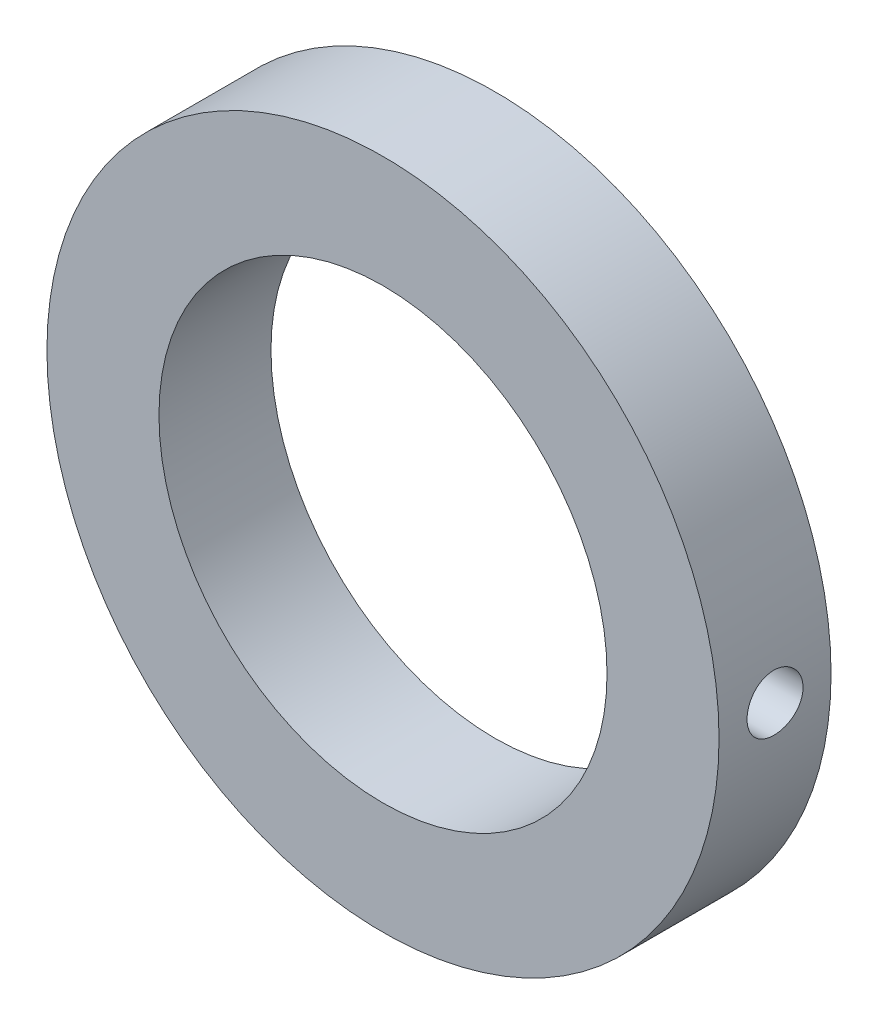
SolidWorks part; units mm, degrees
ref_plane "前视基准面" through (0, 0, 0) normal (0, 0, 1) x (1, 0, 0)
ref_plane "上视基准面" through (0, 0, 0) normal (0, 1, 0) x (1, 0, 0)
ref_plane "右视基准面" through (0, 0, 0) normal (1, 0, 0) x (0, 0, -1)
sketch "草图1" plane through (0, 0, 0) normal (0, 0, 1) x (1, 0, 0)
  circle A0 centre (0, 0) radius 10
  circle A1 centre (0, 0) radius 15
  dimension "D1" = 20
  dimension "D2" = 30
extrude "凸台-拉伸1" add sketch "草图1" along normal blind 5
hole_wizard "M3 螺纹孔2" positions "3D草图2" profile "草图3" tap size "M3" standard "Iso"
sketch3d "3D草图2"
  point P0 (14.9997, 0.1016, 2.5)
sketch "草图3" plane through (14.9997, 0.1016, 2.5) normal (0, 0, 1) x (-0.0068, 1, 0)
  line L0 (0, 0) -> (0, 8.2511)
  line L1 (0, 8.2511) -> (1.25, 7.5)
  line L2 (1.25, 7.5) -> (1.25, 0)
  line L5 (1.25, 0) -> (0, 0)
  line L10 (0, 8.2511) -> (-1.25, 7.5) construction
  line L11 (0, -6.35) -> (0, 107.95) construction
  dimension "螺纹孔钻头直径" = 2.5
  dimension "螺纹孔钻头深度" = 7.5
  dimension "导头角度" = 118
cosmetic thread "孔螺蚊线2" parameters "D1"=5.0784, "D2"=3
